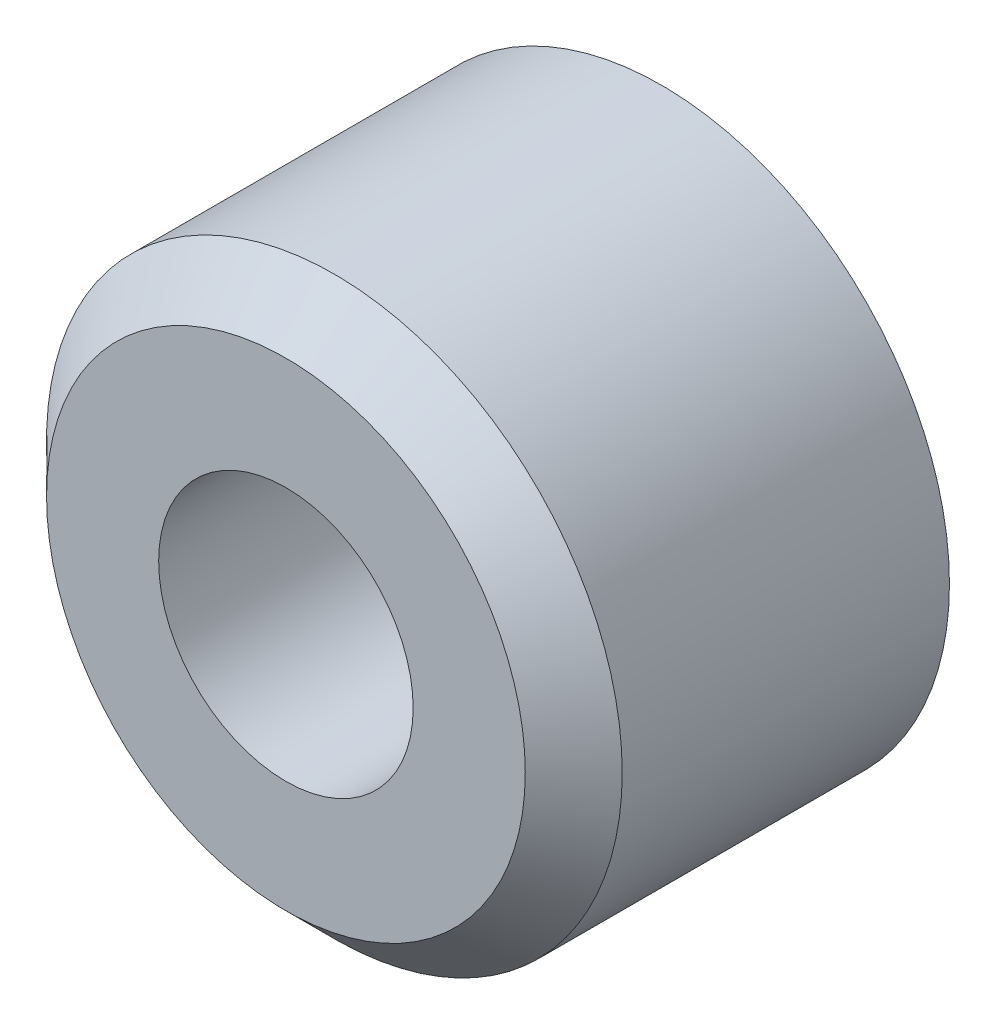
from build123d import *

# Parameters (mm, degrees)
SKETCH_1_R          = 47.5
SKETCH_1_R_2        = 21
EXTRUDE_1_DEPTH     = 62
CHAMFER_1_SIZE      = 8
SKETCH_2_R          = 4
CUT_EXTRUDE_1_DEPTH = 92.413893911
M10X1_0_1_D         = 9
M10X1_0_1_DEPTH     = 10
M10X1_0_1_TIP       = 2.703872786


with BuildPart() as part:
    # 草图1 → 凸台-拉伸1 (new body)
    with BuildSketch(Plane.XY):
        Circle(SKETCH_1_R)
        Circle(SKETCH_1_R_2, mode=Mode.SUBTRACT)
    extrude(amount=EXTRUDE_1_DEPTH)

    # 倒角1
    chamfer_1_edges = [part.edges().sort_by_distance(p)[0] for p in [
        (-47.5, 0, 62),
    ]]
    chamfer(chamfer_1_edges, length=CHAMFER_1_SIZE)

    # 草图2 → 切除-拉伸1 (cut, through all)
    with BuildSketch(Plane(origin=(0, 0, 0), x_dir=(1, 0, 0), z_dir=(0, 1, 0))):
        with Locations(Location((0, -30, 0), (0, 0, 270))):
            Circle(SKETCH_2_R)
    extrude(amount=-CUT_EXTRUDE_1_DEPTH, mode=Mode.SUBTRACT)

    # M10x1.0 螺纹孔1
    with Locations(Plane.XZ.offset(47.5)):
        with Locations((0, 30)):
            Hole(M10X1_0_1_D / 2, depth=M10X1_0_1_DEPTH)
            with Locations((0, 0, -(M10X1_0_1_DEPTH + M10X1_0_1_TIP / 2))):  # 118° drill point
                Cone(0, M10X1_0_1_D / 2, M10X1_0_1_TIP, mode=Mode.SUBTRACT)


solid = part.part
